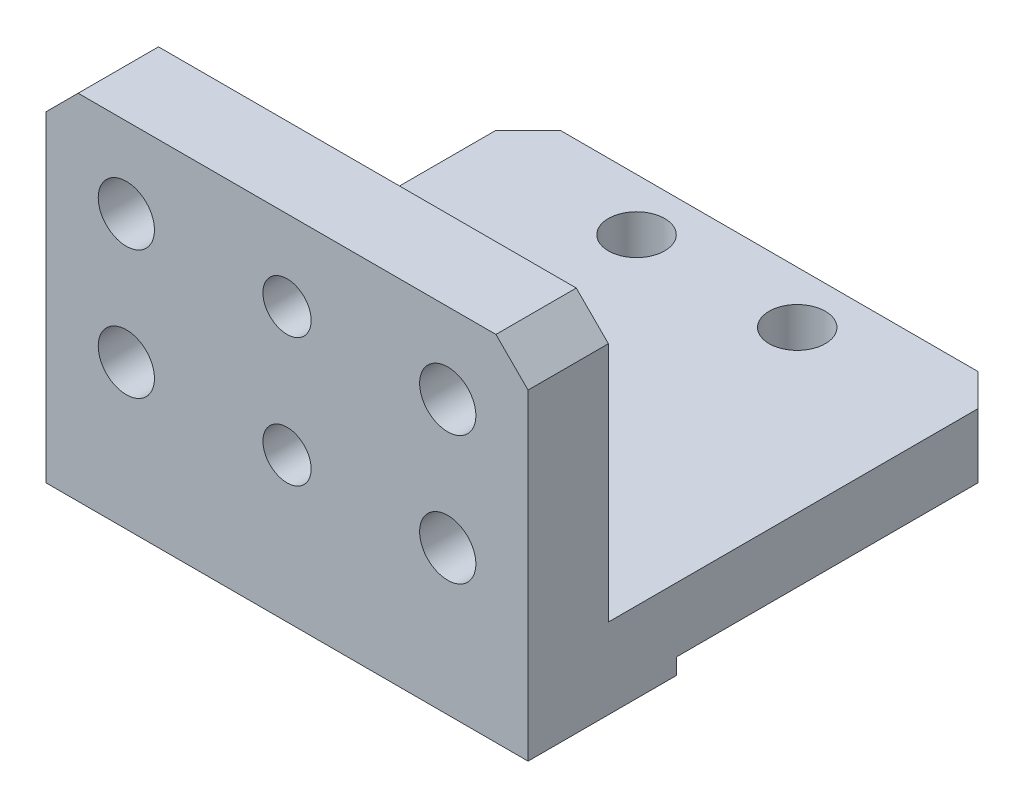
from build123d import *

# Parameters (mm, degrees)
SKETCH_1_W                  = 30
SKETCH_1_H                  = 30
EXTRUDE_1_DEPTH             = 5
SKETCH_2_W                  = 30
SKETCH_2_H                  = 5
EXTRUDE_2_DEPTH             = 17
HOLE_WIZARD_3_5_3_5_1_D     = 3.5
HOLE_WIZARD_3_5_3_5_1_DEPTH = 12.4
HOLE_WIZARD_3_5_3_5_1_TIP   = 1.051506083
SKETCH_5_W                  = 20.75
SKETCH_5_H                  = 1
CUT_EXTRUDE_1_DEPTH         = 41.11234224
CHAMFER_1_SIZE              = 2
HOLE_WIZARD_3_5_3_5_2_D     = 3.5
HOLE_WIZARD_3_5_3_5_2_DEPTH = 12.4
HOLE_WIZARD_3_5_3_5_2_TIP   = 1.051506083
MM_1_D                      = 3
MM_1_DEPTH                  = 12.4
MM_1_TIP                    = 0.901290929


with BuildPart() as part:
    # 草图1 → 凸台-拉伸1 (new body)
    with BuildSketch(Plane(origin=(0, 0, 0), x_dir=(1, 0, 0), z_dir=(0, 1, 0))):
        Rectangle(SKETCH_1_W, SKETCH_1_H)
    extrude(amount=EXTRUDE_1_DEPTH)

    # 草图2 → 凸台-拉伸2 (add)
    with BuildSketch(Plane(origin=(0, 5, 0), x_dir=(1, 0, 0), z_dir=(0, 1, 0))):
        with Locations((0, -12.5)):
            Rectangle(SKETCH_2_W, SKETCH_2_H)
    extrude(amount=EXTRUDE_2_DEPTH)

    # Ø3.5 (3.5) 直径孔1
    with Locations(Plane(origin=(0, 5, 0), x_dir=(1, 0, 0), z_dir=(0, 1, 0))):
        with Locations((-5, 11.75), (5, 11.75), (5, -3.25), (-5, -3.25)):
            Hole(HOLE_WIZARD_3_5_3_5_1_D / 2, depth=HOLE_WIZARD_3_5_3_5_1_DEPTH)
            with Locations((0, 0, -(HOLE_WIZARD_3_5_3_5_1_DEPTH + HOLE_WIZARD_3_5_3_5_1_TIP / 2))):  # 118° drill point
                Cone(0, HOLE_WIZARD_3_5_3_5_1_D / 2, HOLE_WIZARD_3_5_3_5_1_TIP, mode=Mode.SUBTRACT)

    # 草图5 → 切除-拉伸1 (cut, through all)
    with BuildSketch(Plane.ZY.offset(15)):
        with Locations((-4.625, 0.5)):
            Rectangle(SKETCH_5_W, SKETCH_5_H)
    extrude(amount=-CUT_EXTRUDE_1_DEPTH, mode=Mode.SUBTRACT)

    # 倒角1
    chamfer_1_edges = [part.edges().sort_by_distance(p)[0] for p in [
        (-15, 22, 12.5),
        (15, 22, 12.5),
        (-15, 3, -15),
        (15, 3, -15),
    ]]
    chamfer(chamfer_1_edges, length=CHAMFER_1_SIZE)

    # Ø3.5 (3.5) 直径孔2
    with Locations(Plane(origin=(0, 0, 10), x_dir=(-1, 0, 0), z_dir=(0, 0, -1))):
        with Locations((-10, 17), (10, 17), (-10, 9), (10, 9)):
            Hole(HOLE_WIZARD_3_5_3_5_2_D / 2, depth=HOLE_WIZARD_3_5_3_5_2_DEPTH)
            with Locations((0, 0, -(HOLE_WIZARD_3_5_3_5_2_DEPTH + HOLE_WIZARD_3_5_3_5_2_TIP / 2))):  # 118° drill point
                Cone(0, HOLE_WIZARD_3_5_3_5_2_D / 2, HOLE_WIZARD_3_5_3_5_2_TIP, mode=Mode.SUBTRACT)

    # 大小mm 暗销孔1
    with Locations(Plane(origin=(0, 0, 10), x_dir=(-1, 0, 0), z_dir=(0, 0, -1))):
        with Locations((0, 17), (0, 9)):
            Hole(MM_1_D / 2, depth=MM_1_DEPTH)
            with Locations((0, 0, -(MM_1_DEPTH + MM_1_TIP / 2))):  # 118° drill point
                Cone(0, MM_1_D / 2, MM_1_TIP, mode=Mode.SUBTRACT)


solid = part.part
